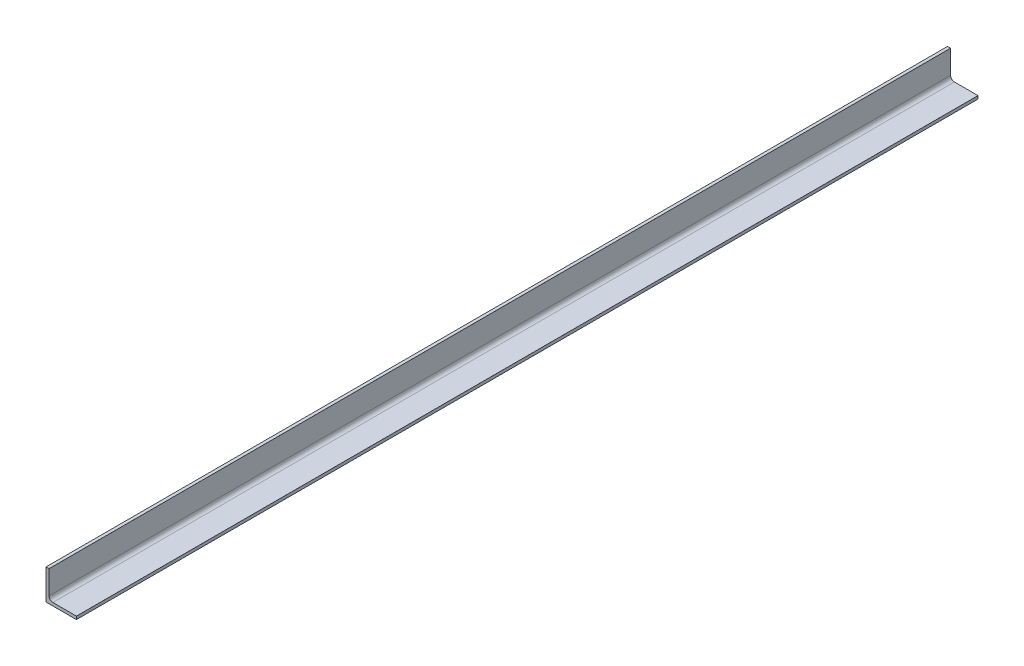
SolidWorks part; units mm, degrees
material "热轧等边角钢 Q235A"
ref_plane "前视基准面" through (0, 0, 0) normal (0, 0, 1) x (1, 0, 0)
ref_plane "上视基准面" through (0, 0, 0) normal (0, 1, 0) x (1, 0, 0)
ref_plane "右视基准面" through (0, 0, 0) normal (1, 0, 0) x (0, 0, -1)
sketch "草图1" plane through (0, 0, 0) normal (0, 0, 1) x (1, 0, 0)
  line L0 (0, 0) -> (0, 40)
  line L1 (0, 40) -> (3.99, 40)
  line L2 (4, 39.99) -> (4, 9)
  line L3 (9, 4) -> (39.99, 4)
  line L4 (40, 3.99) -> (40, 0)
  line L5 (40, 0) -> (0, 0)
  arc A0 (4, 39.99) -> (3.99, 40) centre (3.99, 39.99) ccw
  arc A1 (9, 4) -> (4, 9) centre (9, 9) cw
  arc A2 (40, 3.99) -> (39.99, 4) centre (39.99, 3.99) ccw
  point P9 (4, 40)
  point P14 (40, 4)
extrude "拉伸1" add sketch "草图1" along normal blind 1185
equation "\"D2@草图1\" = \"D1@草图1\""
equation "\"D4@草图1\" = \"D3@草图1\""
equation "\"D7@草图1\" = \"D5@草图1\""
